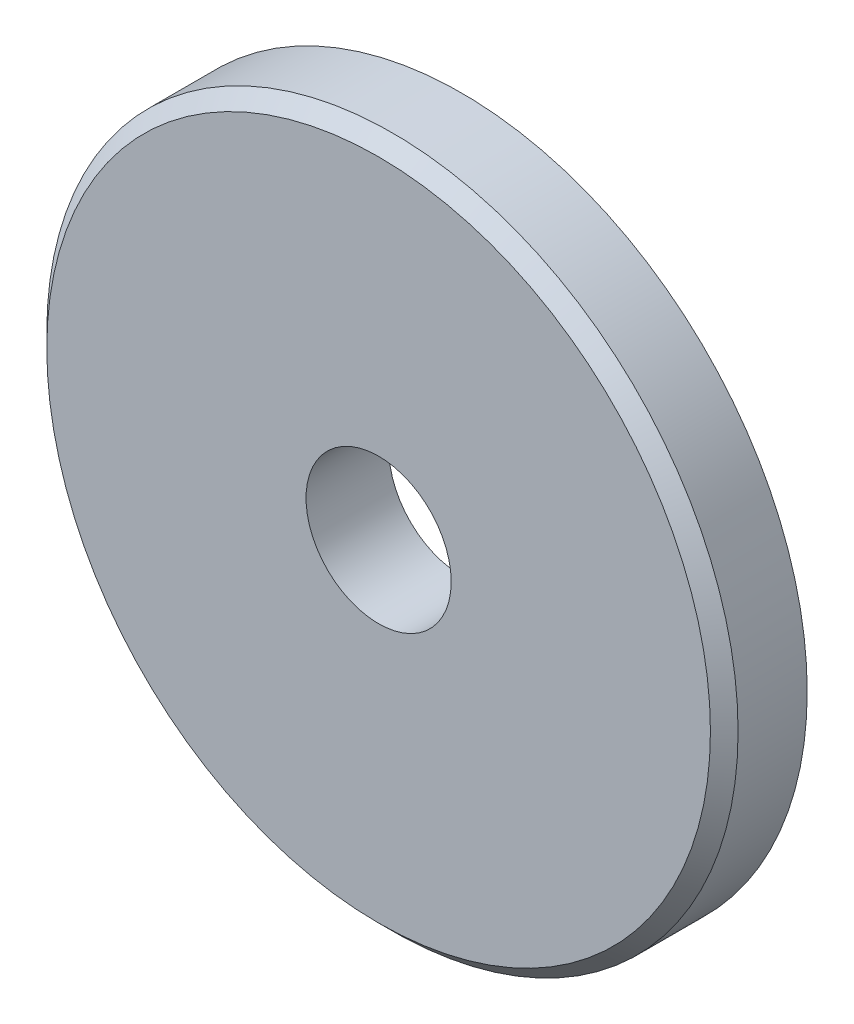
from build123d import *

# Parameters (mm, degrees)
SKETCH_1_R      = 25
SKETCH_1_R_2    = 5.25
EXTRUDE_1_DEPTH = 6
CHAMFER_1_SIZE  = 1


with BuildPart() as part:
    # 草图1 → 凸台-拉伸1 (new body)
    with BuildSketch(Plane.XY):
        Circle(SKETCH_1_R)
        Circle(SKETCH_1_R_2, mode=Mode.SUBTRACT)
    extrude(amount=EXTRUDE_1_DEPTH)

    # 倒角1
    chamfer_1_edges = [part.edges().sort_by_distance(p)[0] for p in [
        (-25, 0, 6),
    ]]
    chamfer(chamfer_1_edges, length=CHAMFER_1_SIZE)


solid = part.part
